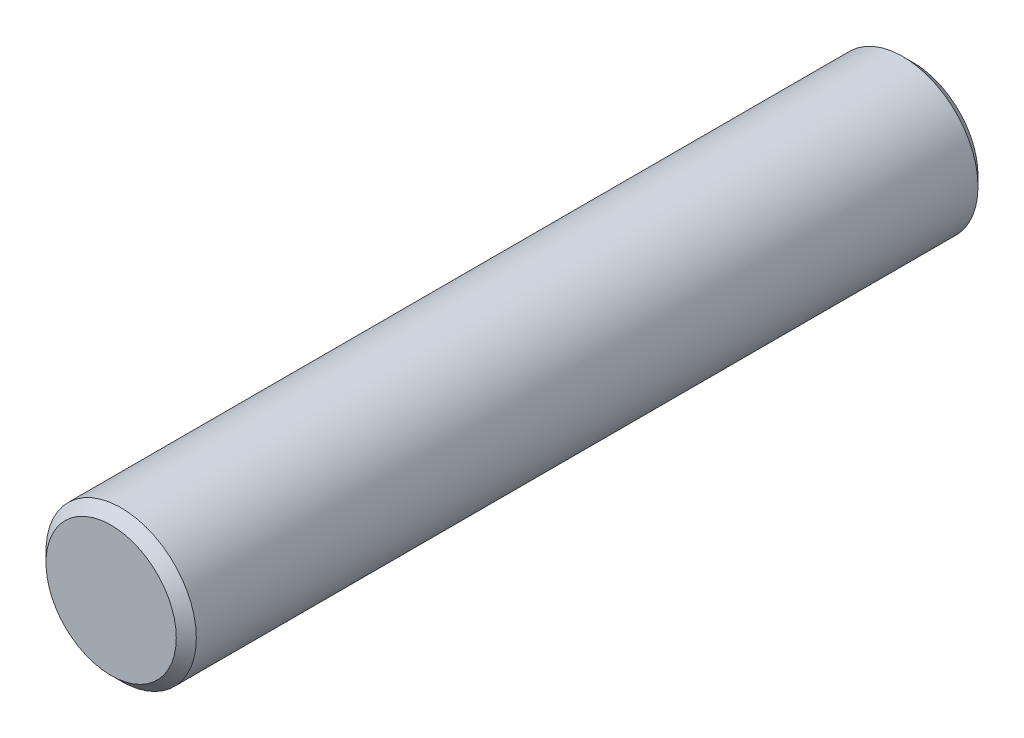
from build123d import *

# Parameters (mm, degrees)
SKETCH1_R           = 1.5
BOSS_EXTRUDE1_DEPTH = 16
CHAMFER1_SIZE       = 0.2


with BuildPart() as part:
    # Sketch1 → Boss-Extrude1 (new body)
    with BuildSketch(Plane.XY):
        Circle(SKETCH1_R)
    extrude(amount=BOSS_EXTRUDE1_DEPTH)

    # Chamfer1
    chamfer1_edges = [part.edges().sort_by_distance(p)[0] for p in [
        (-1.5, 0, 0),
        (-1.5, 0, 16),
    ]]
    chamfer(chamfer1_edges, length=CHAMFER1_SIZE)


solid = part.part
